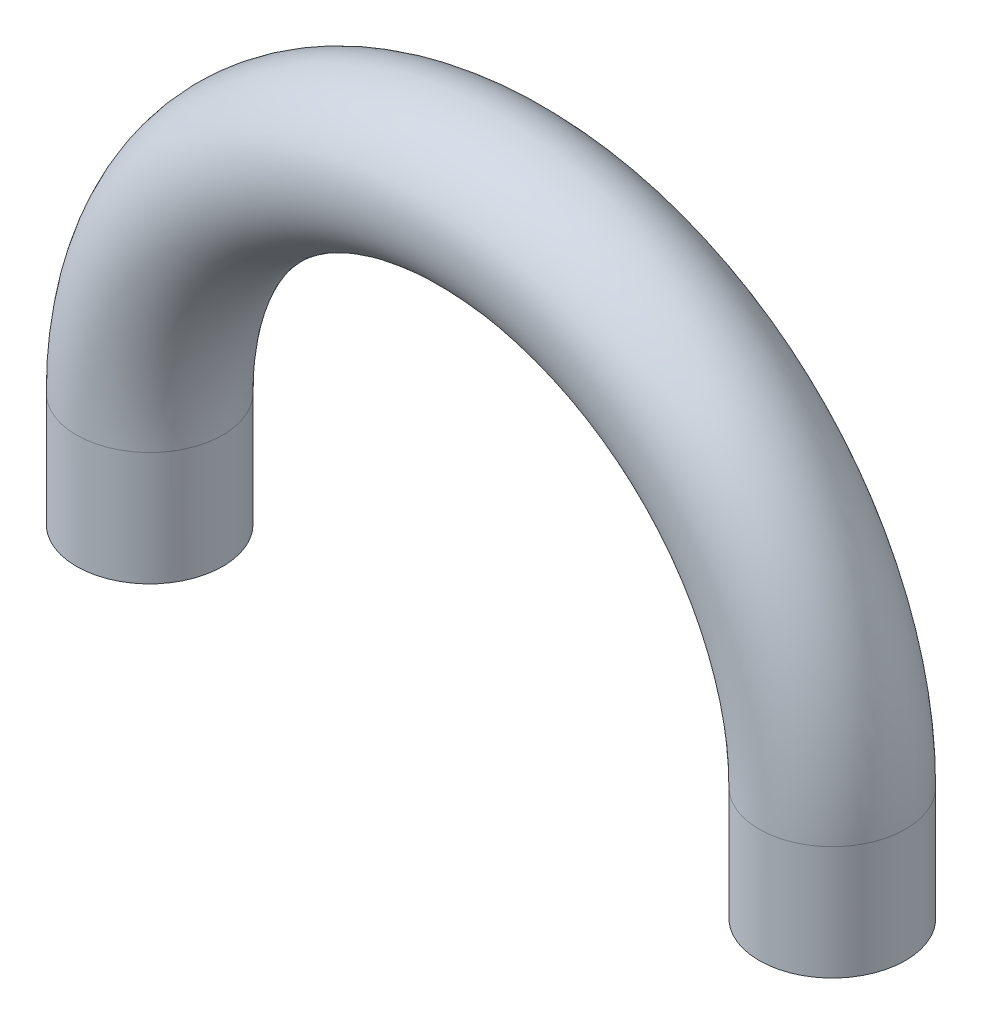
from build123d import *

# Parameters (mm, degrees)
SKETCH4_R = 4.5


with BuildPart() as part:
    # Sweep1: sweep along a path in Sketch1
    with BuildLine(Plane.XY) as sweep1_path:
        Line((-21, -7), (-21, 0))
        ThreePointArc((-21, 0), (0, 21), (21, 0))
        Line((21, 0), (21, -7))
    # Sketch4 → Sweep1 (sweep)
    with BuildSketch(Plane(origin=(0, -7, 0), x_dir=(1, 0, 0), z_dir=(0, 1, 0))):
        with Locations((21, 0)):
            Circle(SKETCH4_R)
    sweep(path=sweep1_path.line)


solid = part.part
